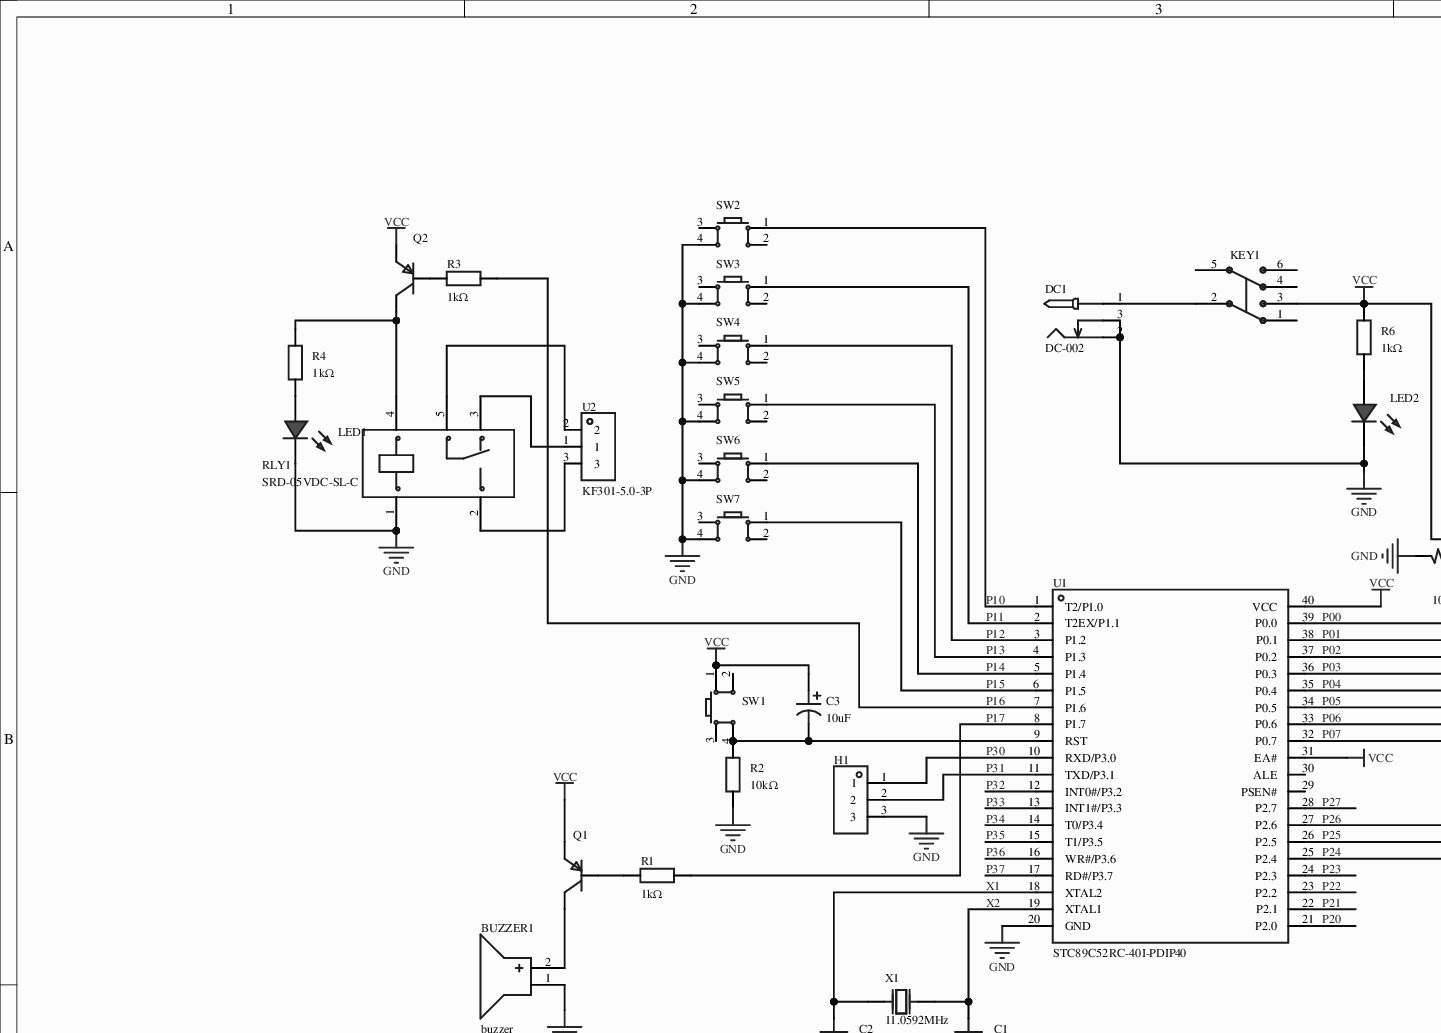
[diagram p0: MISC50235-3.schdoc, top left]
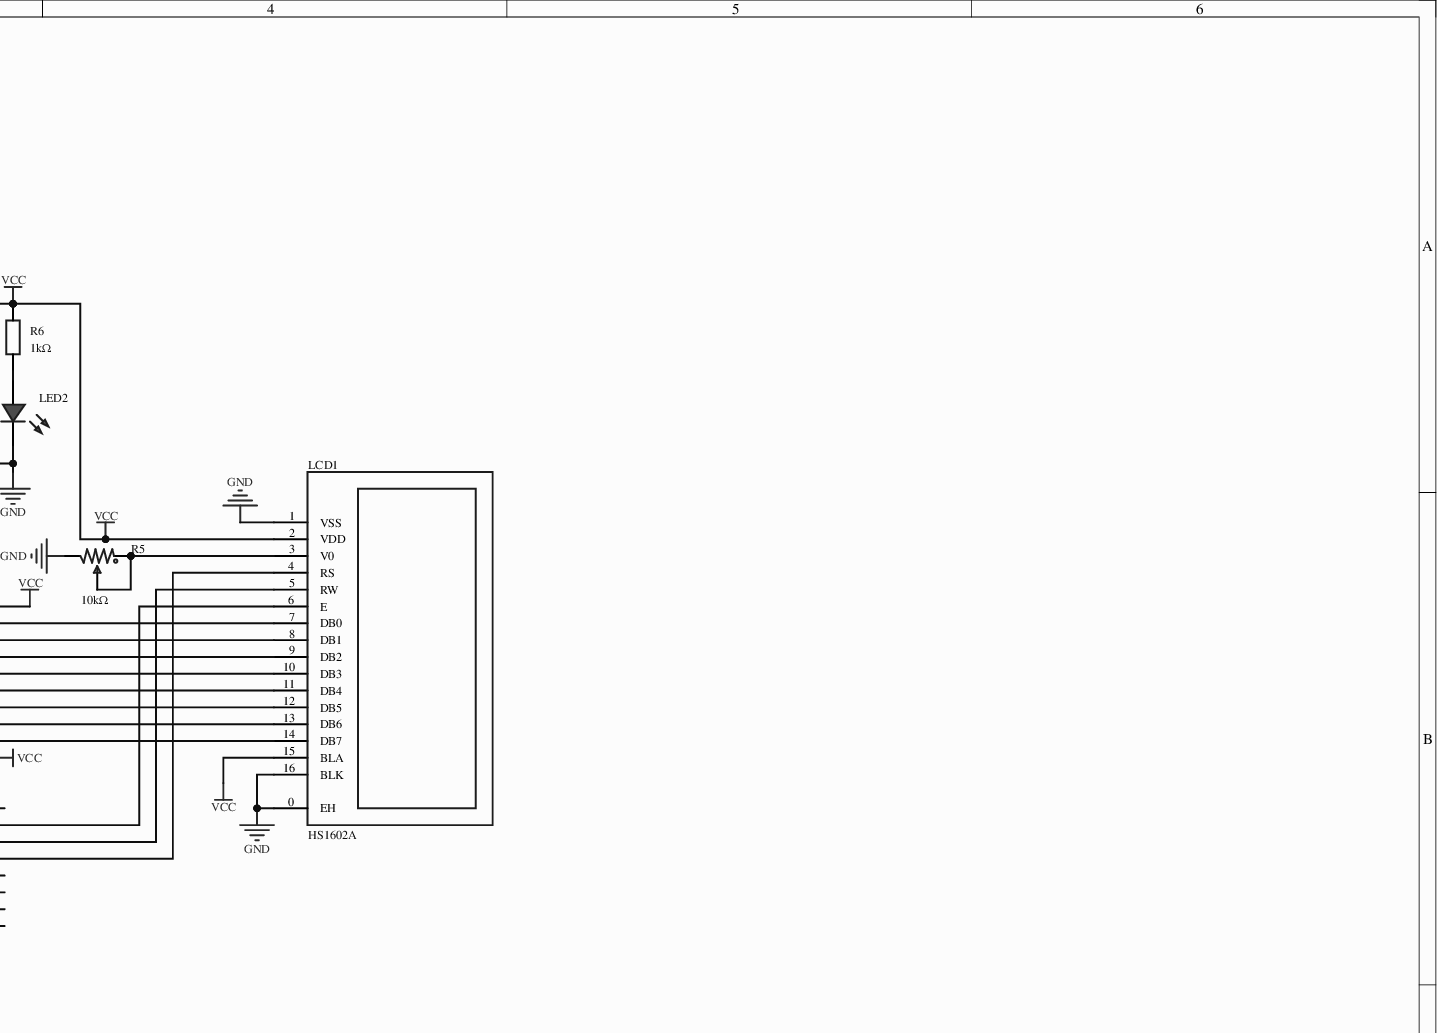
[diagram p1: MISC50235-3.schdoc, top right]
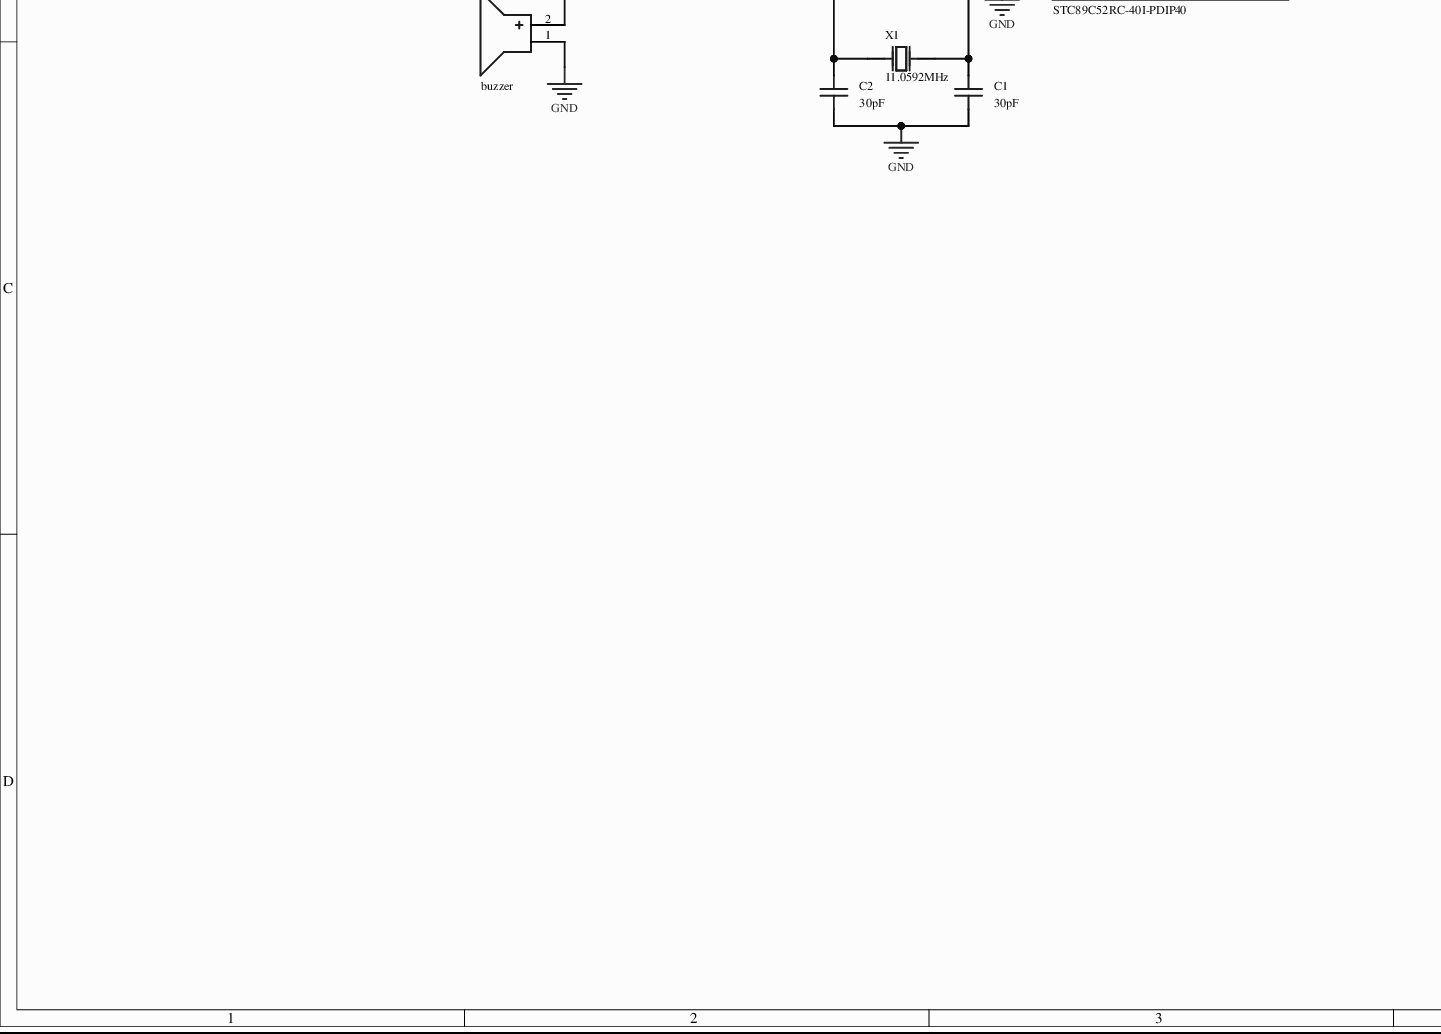
[diagram p2: MISC50235-3.schdoc, bottom left]
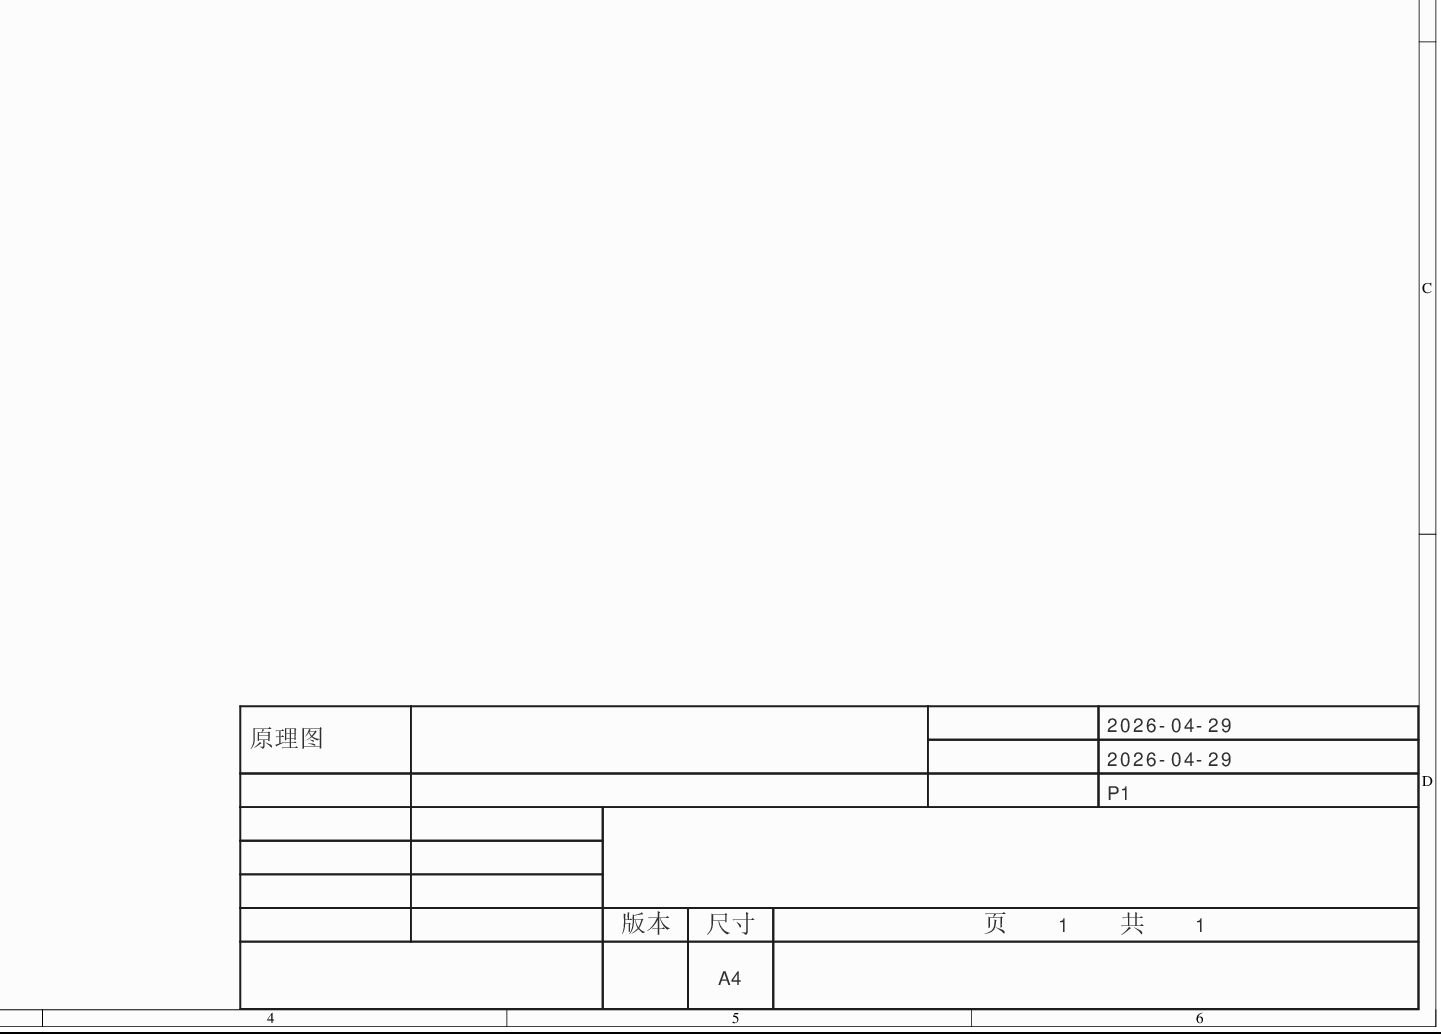
[diagram p3: MISC50235-3.schdoc, bottom right]
# Altium project MISC50235-2.PrjPcb
1 sheet, 29 parts. Net scope: global (net labels, ports and power ports of the same name join across sheets).
Board file: MISC50235.pcbdoc

## Sheet MISC50235-3.schdoc
size 420 x 297 mm; Version: V1.0; @Project Name: MISC50235; @Update Date: 2026-04-29; @Create Date: 2026-04-29; @Board Name: MISC50235; @Create Time: 10:13:01; @Page Count: 1; @Page No: 1; @Schematic Name: MISC50235; @Update Time: 10:13:01; Size: A4

### Parts
BUZZER1  buzzer  [BUZ-TH_BD12.0-P6.00-D0.9-RD]
C1  30pF  [CAP-TH_L3.8-W2.5-P2.54-D0.50]
C2  30pF  [CAP-TH_L3.8-W2.5-P2.54-D0.50]
C3  10uF  [CAP-TH_BD5.0-P2.00-D0.8-FD-10UF50VC110GL]
DC1  DC-002  [DC-IN-TH_DC-3510]
H1  (no value)  [HDR-TH_3P-P2.54-V-M]
KEY1  无自锁开关 8.5×8.5 无声  [SW-TH_6P-L8.5-W8.5-P2.54]  (value not drawn)
LCD1  HS1602A  [LCD1602]
LED1  (no value)  [LED_TH-3mm]
LED2  (no value)  [LED_TH-3mm]
Q1  (no value)  [S8550P_TO-92]
Q2  (no value)  [S8550P_TO-92]
R1  1kΩ  [Res_1/8W]
R2  10kΩ  [Res_1/8W]
R3  1kΩ  [Res_1/8W]
R4  1kΩ  [Res_1/8W]
R5  10kΩ  [RES-ADJ-SMD_RM065-V1]
R6  1kΩ  [Res_1/8W]
RLY1  SRD-05VDC-SL-C  [RELAY-TH_SRD-XXVDC-XL-C]
SW1  (no value)  [SW-TH_4P-L6.0-W6.0-P4.50-LS6.5]
SW2  (no value)  [SW-TH_4P-L6.0-W6.0-P4.50-LS6.5]
SW3  (no value)  [SW-TH_4P-L6.0-W6.0-P4.50-LS6.5]
SW4  (no value)  [SW-TH_4P-L6.0-W6.0-P4.50-LS6.5]
SW5  (no value)  [SW-TH_4P-L6.0-W6.0-P4.50-LS6.5]
SW6  (no value)  [SW-TH_4P-L6.0-W6.0-P4.50-LS6.5]
SW7  (no value)  [SW-TH_4P-L6.0-W6.0-P4.50-LS6.5]
U1  STC89C52RC-40I-PDIP40  [DIP-40_L52.0-W13.7-P2.54-LS15.2-BL]
U2  KF301-5.0-3P  [CONN-TH_3P-P5.00_KF301-5.0-3P]
X1  11.0592MHz  [OSC-TH_L11.1-W4.7-P4.88]

### Nets
GND: BUZZER1.1(-) C1.1 C2.1 DC1.2 DC1.3 H1.3 LCD1.0(EH) LCD1.1(VSS) LCD1.16(BLK) LED1.2(A) LED2.2(A) R2.1 R5.3 RLY1.1 SW2.4 SW3.4 SW4.4 SW5.4 SW6.4 SW7.4 U1.20(GND)
VCC: C3.1 KEY1.3 LCD1.2(VDD) LCD1.15(BLA) Q1.1(E) Q2.1(E) R6.2 SW1.1 U1.31(EA#) U1.40(VCC)
P00: LCD1.7(DB0) U1.39(P0.0)
P01: LCD1.8(DB1) U1.38(P0.1)
P02: LCD1.9(DB2) U1.37(P0.2)
P03: LCD1.10(DB3) U1.36(P0.3)
P04: LCD1.11(DB4) U1.35(P0.4)
P05: LCD1.12(DB5) U1.34(P0.5)
P06: LCD1.13(DB6) U1.33(P0.6)
P07: LCD1.14(DB7) U1.32(P0.7)
P10: SW2.1 U1.1(T2/P1.0)
P11: SW3.1 U1.2(T2EX/P1.1)
P12: SW4.1 U1.3(P1.2)
P13: SW5.1 U1.4(P1.3)
P14: SW6.1 U1.5(P1.4)
P15: SW7.1 U1.6(P1.5)
P16: R3.2 U1.7(P1.6)
P17: R1.2 U1.8(P1.7)
P20: U1.21(P2.0)
P21: U1.22(P2.1)
P22: U1.23(P2.2)
P23: U1.24(P2.3)
P24: LCD1.4(RS) U1.25(P2.4)
P25: LCD1.5(RW) U1.26(P2.5)
P26: LCD1.6(E) U1.27(P2.6)
P27: U1.28(P2.7)
P30: H1.1 U1.10(RXD/P3.0)
P31: H1.2 U1.11(TXD/P3.1)
P32: U1.12(INT0#/P3.2)
P33: U1.13(INT1#/P3.3)
P34: U1.14(T0/P3.4)
P35: U1.15(T1/P3.5)
P36: U1.16(WR#/P3.6)
P37: U1.17(RD#/P3.7)
X1: C2.2 U1.18(XTAL2) X1.1(OSC1)
X2: C1.2 U1.19(XTAL1) X1.2(OSC2)
NetBUZZER1_2: BUZZER1.2(+) Q1.3(C)
NetC3_2: C3.2 R2.2 SW1.4 U1.9(RST)
NetDC1_1: DC1.1 KEY1.2
NetLCD1_3: LCD1.3(V0) R5.1 R5.2
NetLED1_1: LED1.1(C) R4.1
NetLED2_1: LED2.1(C) R6.1
NetQ1_2: Q1.2(B) R1.1
NetQ2_2: Q2.2(B) R3.1
NetQ2_3: Q2.3(C) R4.2 RLY1.4
NetRLY1_2: RLY1.2 U2.3
NetRLY1_3: RLY1.3 U2.1
NetRLY1_5: RLY1.5 U2.2

Not connected (* = marked no-connect by the designer): KEY1 1 4 5 6; SW1 2 3; SW2 2 3; SW3 2 3; SW4 2 3; SW5 2 3; SW6 2 3; SW7 2 3; U1 29(PSEN#)* 30(ALE)*

### Notes on the sheet
- 2026-04-29
- 原理图
- P1
- 版本
- 尺寸
- A4
- 页    1    共    1

### Library data of the parts
BUZZER1 = buzzer: AddInBom: yes; ModelId: af17e4151ed84fc2a628230bf23763630819f05c4eef4c71ace90d822a990e87; ModelTransform: 472.44,472.176,0,270,0,0,0,0,-196.85; Symbol: BUZZER; Device: buzzer; LCSC Part Name: buzzer; SupplierPart: C9900014030; ManufacturerPart: buzzer; Supplier Footprint: buzzer; JLCPCB Part Class: Extended Part; Supplier: LCSC; ConvertToPcb: yes; FootprintName: BUZ-TH_BD12.0-P6.00-D0.9-RD; ModelName: BUZ-TH_BD12.0-P6.00-D0.9-RD
C1 C2 = C315C300K3G5TA7301: 容值:30pF;精度:±10%;额定电压:25V;温度系数:C0G;; Manufacturer: KEMET(基美); AddInBom: yes; ModelId: 0be8c650c9044d099e9add656cc6dda60819f05c4eef4c71ace90d822a990e87; ModelTransform: 149.606,98.8187,0,0,0,0,0,0,-196.85; Tolerance: ±10%; Voltage Rating: 25V; Temperature Coefficient: C0G; Pin Spacing: 2.54mm; Symbol: C315C300K3G5TA7301; Device: C315C300K3G5TA7301; LCSC Part Name: 30pF ±10% 25V; SupplierPart: C2245291; ManufacturerPart: C315C300K3G5TA7301; Supplier Footprint: 插件,P=2.54mm; JLCPCB Part Class: Extended Part; Datasheet: https://item.szlcsc.com/datasheet/C315C300K3G5TA7301/2337370.html; Supplier: LCSC; ConvertToPcb: yes; FootprintName: CAP-TH_L3.8-W2.5-P2.54-D0.50; ModelName: CAP-TH_L3.8-W2.5-P2.54-D0.50; Value: 30pF
C3 = 10UF50VC110GL: 容值:10uF;精度:±20%;额定电压:50V;纹波电流:120mA@100KHz;等效串联电阻(ESR):1.6Ω;; Manufacturer: Econd(米朗电子); AddInBom: yes; Tolerance: ±20%; Voltage Rating: 50V; Equivalent Series Resistance(ESR): 1.6Ω; Pin Spacing: 2mm; Lifetime: 5000hrs@105℃; Symbol: 10UF50VC110GL; Device: 10UF50VC110GL; LCSC Part Name: 10uF ±20% 50V; SupplierPart: C46867109; ManufacturerPart: 10UF50VC110GL; Supplier Footprint: 插件,D5xL11mm; JLCPCB Part Class: Extended Part; Datasheet: https://item.szlcsc.com/datasheet/10UF50VC110GL/49031974.html; Supplier: LCSC; ConvertToPcb: yes; FootprintName: CAP-TH_BD5.0-P2.00-D0.8-FD-10UF50VC110GL; Value: 10uF; Ripple Current: 120mA@100KHz; Diameter: 5mm; Height - Seated (Max): 11mm; Operating Temperature: -40℃~+105℃
DC1 = DC-002: AddInBom: yes; ModelId: 28059cb5f325411c86e5e1af88d5b1310819f05c4eef4c71ace90d822a990e87; ModelTransform: 450.787,208.661,0,180,0,0,113.189,-47.244,-125.984; Symbol: DC-002; Device: DC-002; LCSC Part Name: DC-002 铁脚 内铁芯1.0mm; SupplierPart: C12568; ManufacturerPart: DC-002; Supplier Footprint: 插件; JLCPCB Part Class: Extended Part; Supplier: LCSC; ConvertToPcb: yes; FootprintName: DC-IN-TH_DC-3510; ModelName: DC-IN-TH_DC-3510
H1 = HDR-M_2.54_1x3P: AddInBom: yes; ModelId: bb473b6d38ff42a99216a4fcdbdcc4cb0819f05c4eef4c71ace90d822a990e87; ModelName: HDR-TH_3P-P2.54-M-LI-1X3P; ModelTransform: 300.03877,100,0,0,0,0,0,0,-118.11; Symbol: HDR-M_2.54_1x3P; Device: HDR-M_2.54_1x3P; ConvertToPcb: yes; FootprintName: HDR-TH_3P-P2.54-V-M; SupplierPart: C2937625; Supplier Footprint: 插件
KEY1 = 无自锁开关 8.5×8.5 无声: 6脚，8.5×8.5; Symbol: No self-locking switch 8.5×8.5 silent; AddInBom: yes; ModelId: 4c72b3966b92446eb355e1bd0fb4f8800819f05c4eef4c71ace90d822a990e87; ModelTransform: 342.519,334.645,0,180,0,0,0,0,-137.795; Device: 无自锁开关 8.5×8.5 无声; LCSC Part Name: 无自锁开关 8.5×8.5  无声; SupplierPart: C26228; ManufacturerPart: 无自锁开关 8.5×8.5 无声; Supplier Footprint: 插件; JLCPCB Part Class: Extended Part; Supplier: LCSC; ConvertToPcb: yes; FootprintName: SW-TH_6P-L8.5-W8.5-P2.54; ModelName: SW-TH_6P-L8.5-W8.5-P2.54
LCD1 = HS1602A: 主控芯片:SPLC780;尺寸(inch):2;; Manufacturer: HS(汉昇); AddInBom: yes; ModelId: f9d832f46a914cadb50fc4d4cefd25170819f05c4eef4c71ace90d822a990e87; ModelTransform: 3149.6,1417.32,0,0,0,0,0,0,-118.11; Symbol: HS1602A; Device: HS1602A; LCSC Part Name: 2.0寸16*2单色字符字符液晶显示屏; SupplierPart: C5329588; ManufacturerPart: HS1602A; Supplier Footprint: -; JLCPCB Part Class: Extended Part; Datasheet: https://atta.szlcsc.com/upload/public/pdf/source/20221212/35734F14DBB323F90DD8DBE1717CD9FD.pdf; Supplier: LCSC; ConvertToPcb: yes; FootprintName: LCD1602; ModelName: LCD1602; Main Control Chip: SPLC780; Size: 2; Operating Temperature: -20℃~+70℃
LED1 LED2 = LED_TH-R_3mm: ConvertToPcb: yes; ModelId: a497c992633541038a38947cdc58012f0819f05c4eef4c71ace90d822a990e87; ModelName: LED-TH-3mm_R; ModelTransform: 141.274,153.327,0,0,0,0,-5.984,0,-137.795; Symbol: LED_TH-R; Device: LED_TH-R_3mm; AddInBom: yes; FootprintName: LED_TH-3mm; Supplier Footprint: 插件
Q1 Q2 = S8550_TO_PNP: ConvertToPcb: yes; ModelId: aafe8e06f2154e7c93506efd0d6632dd0819f05c4eef4c71ace90d822a990e87; ModelName: TO-92-3_L4.9-W3.7-P1.27-L; ModelTransform: 180.78,141.44,417.3,0,0,0,0,0,-200; Symbol: S8550_TO_PNP; Device: S8550_TO_PNP; AddInBom: yes; Supplier Footprint: TO-92; FootprintName: S8550P_TO-92
R1-R4 R6 = Res_AXIAL-1/8W: Symbol: 电阻; ConvertToPcb: yes; ModelId: b2b5ae7ae4c642178fe0039925c86a3f0819f05c4eef4c71ace90d822a990e87; ModelName: RES-TH_BD1.8-L3.2-P7.20-D0.4; ModelTransform: 282.86,66.88,253.09,0,0,0,0,0,-191; Device: Res_AXIAL-1/8W; AddInBom: yes; Supplier Footprint: 轴向引线; FootprintName: Res_1/8W
  R1 R3 R4 R6: Value: 1kΩ
  R2: Value: 10kΩ
R5 = RM065-103(10K): 阻值:10kΩ;精度:±25%;功率:100mW;; Manufacturer: BOCHEN(博晨); AddInBom: yes; ModelId: c816c2b7942147f5a832150e8ef6960c0819f05c4eef4c71ace90d822a990e87; ModelTransform: 255.905,283.464,0,0,0,0,0.025,-3.937,-157.48; Tolerance: ±25%; Voltage Rating: 50V; Power(Watts): 100mW; Symbol: RM065-103(10K); Device: RM065-103(10K); LCSC Part Name: 10kΩ ±25%; SupplierPart: C5205021; ManufacturerPart: RM065-103(10K); Supplier Footprint: 插件,7.3x6.4mm; JLCPCB Part Class: Extended Part; Datasheet: https://item.szlcsc.com/datasheet/RM065-103(10K)/5896379.html; Supplier: LCSC; ConvertToPcb: yes; FootprintName: RES-ADJ-SMD_RM065-V1; ModelName: RES-ADJ-SMD_RM065-V1; Value: 10kΩ
RLY1 = SRD-05VDC-SL-C: 线圈电压:5V;触点形式:一组转换:1C(单刀双掷-转换);触点容量(电阻负载):-;最大切换电压:250V@AC;最大切换电流:15A;; Manufacturer: 松乐; AddInBom: yes; ModelId: d0eda9b8bf8746d18ae810ab88dc78e70819f05c4eef4c71ace90d822a990e87; ModelName: RELAY-TH_L19.2-W15.6-H15.8; ModelTransform: 755.904,622.4397,0,0,0,0,34.882,0,-118.11; Coil Voltage: 5V; Coil Rated Power: 360mW; Switching Current(Max): 15A; Coil Type: 无极性-单线圈; Coil Resistance: 70Ω; Contact Resistance: 100mΩ; Operate Time: 10ms; Symbol: SRD-05VDC-SL-C; Device: SRD-05VDC-SL-C; LCSC Part Name: 蓝色 单组转换型继电器; SupplierPart: C35449; ManufacturerPart: SRD-05VDC-SL-C; Supplier Footprint: 插件,19.2x15.6mm; JLCPCB Part Class: Extended Part; Datasheet: https://item.szlcsc.com/datasheet/SRD-05VDC-SL-C/36422.html; Supplier: LCSC; ConvertToPcb: yes; FootprintName: RELAY-TH_SRD-XXVDC-XL-C; Contact Form: 一组转换:1C(单刀双掷-转换); Number of Pins: 5; Contact Rating: -; Switching Voltage(Max): 250V@AC; Release Time: 10ms
SW1-SW7 = Key_TH_6x6x6: 触点电流:50mA;额定电压(DC):12V;绝缘电阻:100MΩ;电路结构:单刀单掷;安装方式:直插;按钮形状:圆形按钮;按钮/盖帽颜色:黑色;作用力:260gf@±30gf;工作温度:-25℃~+70℃;引脚样式:PC引脚;开关长度:6mm;开关宽度:6mm;开关高度:6mm;带支架:否;; Symbol: 轻触按键; AddInBom: yes; ModelId: 20eee248bc684ccd8cbdbb1d0d91ec6f0819f05c4eef4c71ace90d822a990e87; ModelName: SW-TH_4P-L6.0-W6.0-H5.0-LS6.5-P4.50; ModelTransform: 236.22,323.03,0,90,0,0,0,0,-137.795; Device: Key_TH_6x6x6; ConvertToPcb: yes; FootprintName: SW-TH_4P-L6.0-W6.0-P4.50-LS6.5; Supplier Footprint: 插件
U1 = STC89C52RC-40I-PDIP40: CPU内核:51家族;CPU最大主频:-;; Manufacturer: STC; AddInBom: yes; ModelId: 16d4686a009b4ddca948f91eddb57b140819f05c4eef4c71ace90d822a990e87; ModelName: DIP-40_L52.3-W13.8-H4.0-LS15.24-P2.54; ModelTransform: 2059.051,615.743,0,0,0,0,0,0,-118.11; CPU Core: 51家族; Program Storage Size: 8KB; Program Memory Type: FLASH; Voltage - Supply: 3.3V~5.5V; Symbol: STC89C52RC-40I; Device: STC89C52RC-40I-PDIP40; LCSC Part Name: 单片机原理及应用; SupplierPart: C14022; ManufacturerPart: STC89C52RC-40I-PDIP40; Supplier Footprint: DIP-40; JLCPCB Part Class: Extended Part; Datasheet: https://item.szlcsc.com/datasheet/STC89C52RC-40I-PDIP40/14679.html; Supplier: LCSC; ConvertToPcb: yes; FootprintName: DIP-40_L52.0-W13.7-P2.54-LS15.2-BL; CPU Maximum Speed: -; RAM Size: -; EEPROM: -; Number of I/O: -; ADC (Bit): -; DAC (Bit): -
U2 = KF301-5.0-3P: 结构:1x3P;间距:5mm;颜色:蓝色;安装方式:直插;排数:1;每排PIN数:3;额定电流:17A;额定电压:250V;线规 - AWG:14~22;线规 - 平方毫米:1.5;工作温度:-30℃~+120℃;; Manufacturer: KEFA(科发); AddInBom: yes; ModelId: 7a1c767a6883477d8097e3100aeff3430819f05c4eef4c71ace90d822a990e87; ModelTransform: 606.298,303.149,0,0,0,0,7.874,5.905,-165.354; Number of Positions or Pins: 1x3P; Pitch: 5mm; Number of PINs Per Row: 3; Current Rating: 17A; Voltage Rating (Max): 250V; Wire Gauge - AWG: 14~22; Wire Gauge - mm2: 1.5; Symbol: KF301-5.0-3P; Device: KF301-5.0-3P; LCSC Part Name: 1x3P 5mm 直插 排数:1 每排P数:3; SupplierPart: C474882; ManufacturerPart: KF301-5.0-3P; Supplier Footprint: 插件,P=5mm; JLCPCB Part Class: Extended Part; Datasheet: https://item.szlcsc.com/datasheet/KF301-5.0-3P/481500.html; Supplier: LCSC; ConvertToPcb: yes; FootprintName: CONN-TH_3P-P5.00_KF301-5.0-3P; ModelName: CONN-TH_3P-P5.00_KF301-5.0-3P; Color: 蓝色; Mounting Type: 直插; Number of Pins: 3P; Number of Rows: 1; Operating Temperature: -30℃~+120℃
X1 = 9AC11059302060C3: 晶振类型:直插晶振;频率:11.0592MHz;常温频差:±20ppm;负载电容:30pF;; Manufacturer: JGHC(晶光华); AddInBom: yes; ModelId: f2ed30de83344a4b83b1c4b1b9fe18560819f05c4eef4c71ace90d822a990e87; ModelTransform: 436.37503,185.039,0,0,0,0,0,0,-137.795; Normal temperature Frequency Tolerance: ±20ppm; Load Capacitance: 30pF; Equivalent Series Resistance(ESR): 60Ω; Symbol: 9AC11059302060C3; Device: 9AC11059302060C3; LCSC Part Name: 11.0592MHz ±20ppm 30pF; SupplierPart: C2715911; ManufacturerPart: 9AC11059302060C3; Supplier Footprint: HC-49S; JLCPCB Part Class: Extended Part; Datasheet: https://item.szlcsc.com/datasheet/9AC11059302060C3/2832137.html; Supplier: LCSC; ConvertToPcb: yes; FootprintName: OSC-TH_L11.1-W4.7-P4.88; ModelName: OSC-TH_L11.1-W4.7-P4.88; Type: 直插晶振; Value: 11.0592MHz; Operating Temperature: -40℃~+85℃